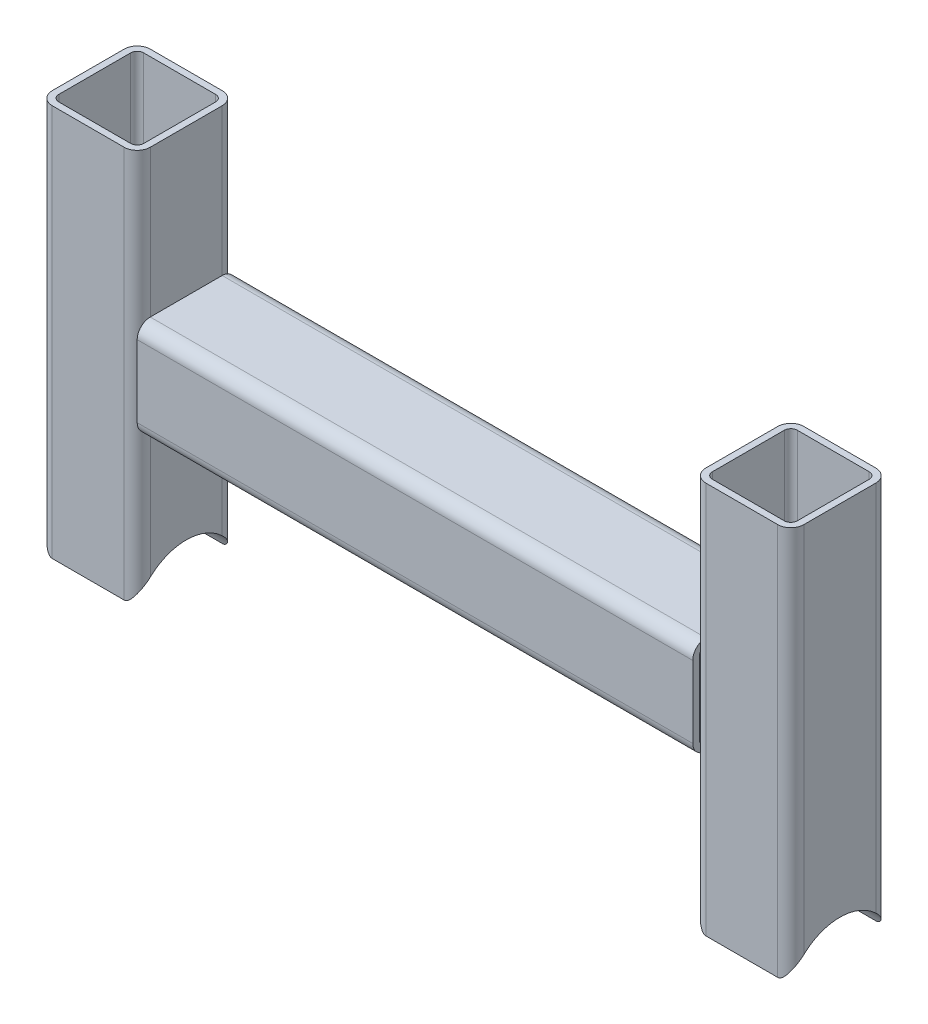
SolidWorks part; units mm, degrees
material "Q235B"
ref_plane "Front Plane" through (0, 0, 0) normal (0, 0, 1) x (1, 0, 0)
ref_plane "Top Plane" through (0, 0, 0) normal (0, 1, 0) x (1, 0, 0)
ref_plane "Right Plane" through (0, 0, 0) normal (1, 0, 0) x (0, 0, -1)
sketch "草图1" plane through (0, 0, 0) normal (0, 0, 1) x (1, 0, 0)
  line L0 (100, 0) -> (-100, 0)
  line L1 (-100, -60) -> (-100, 60)
  line L2 (100, -60) -> (100, 60)
  point P4 (0, 0)
  point P8 (-100, 0)
  point P11 (100, 0)
  dimension "D1" = 200
  dimension "D2" = 120
other "Gb／t 6728—2002 Square hollow section steel 30×2-example.com(1)"
ref_plane "Plane1" through (-100, -60, 0) normal (0, 1, 0) x (-1, 0, 0)
sketch "Sketch1" plane through (-100, -60, 0) normal (0, 1, 0) x (-1, 0, 0)
  line L0 (-11, -13) -> (11, -13)
  line L1 (-13, -11) -> (-13, 11)
  line L2 (11, 13) -> (-11, 13)
  line L3 (13, 11) -> (13, -11)
  line L4 (-11, -15) -> (11, -15)
  line L5 (-15, -11) -> (-15, 11)
  line L6 (11, 15) -> (-11, 15)
  line L7 (15, 11) -> (15, -11)
  arc A0 (15, 11) -> (11, 15) centre (11, 11) ccw
  arc A1 (11, -15) -> (15, -11) centre (11, -11) ccw
  arc A2 (-15, -11) -> (-11, -15) centre (-11, -11) ccw
  arc A3 (-11, 15) -> (-15, 11) centre (-11, 11) ccw
  arc A4 (-11, 13) -> (-13, 11) centre (-11, 11) ccw
  arc A5 (13, 11) -> (11, 13) centre (11, 11) ccw
  arc A6 (11, -13) -> (13, -11) centre (11, -11) ccw
  arc A7 (-13, -11) -> (-11, -13) centre (-11, -11) ccw
  point P0 (-15, 0)
  point P1 (15, 0)
  point P2 (0, 15)
  point P3 (0, -15)
  point P4 (0, 0)
  point P5 (-15, -15)
  point P6 (15, -15)
  point P7 (15, 15)
  point P8 (-15, 15)
  point P33 (0, 0)
  dimension "D1" = 4
  dimension "Thickness" = 2
  dimension "V_leg" = 30
sketch "Sketch3" plane through (0, 0, 0) normal (1, 0, 0) x (0, 0, -1)
  line L1 (0, -65.5678) -> (0, -60) construction
  line L2 (-11, -60) -> (11, -60) construction
  circle A0 centre (0, -65.5678) radius 16
  dimension "D1" = 32
extrude "Cut-Extrude1" cut sketch "Sketch3" against normal through all both and the other way through all
